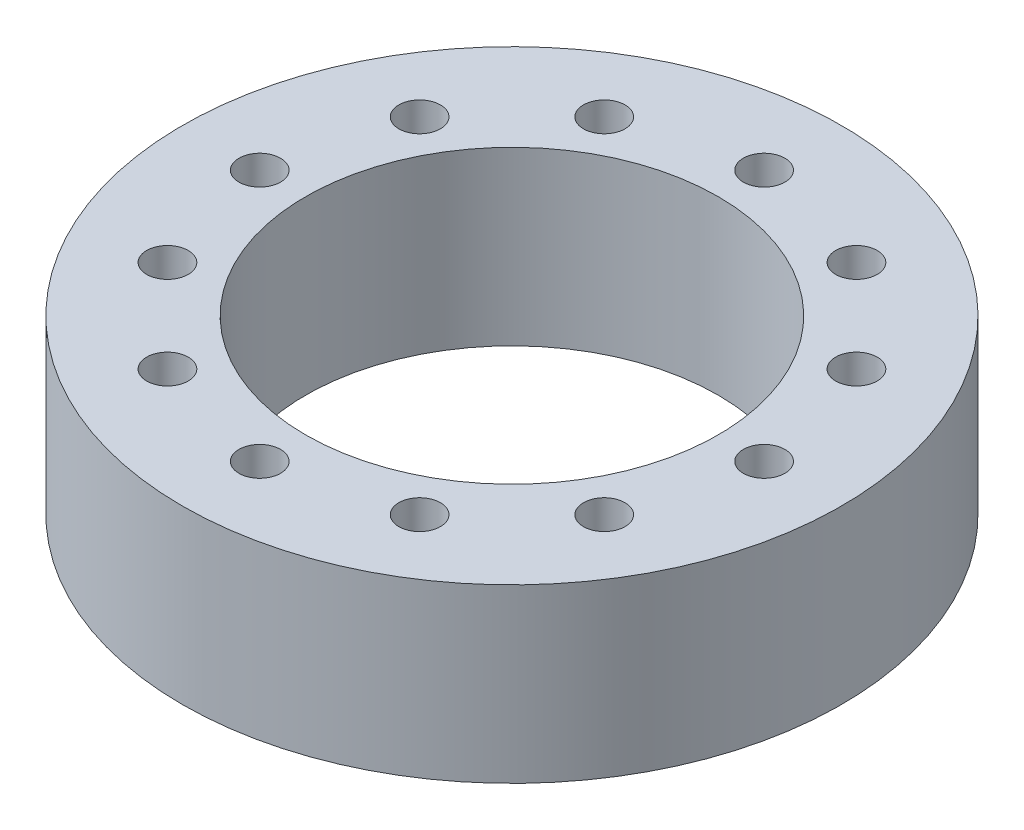
from build123d import *

# Parameters (mm, degrees)
SKETCH1_R           = 115
SKETCH1_R_2         = 72
SKETCH1_R_3         = 7.25
BOSS_EXTRUDE1_DEPTH = 60
SKETCH2_R           = 11
CUT_EXTRUDE1_DEPTH  = 30


with BuildPart() as part:
    # Sketch1 → Boss-Extrude1 (new body)
    with BuildSketch(Plane(origin=(0, 0, 0), x_dir=(1, 0, 0), z_dir=(0, 1, 0))):
        with Locations(Location((0, 0, 0), (0, 0, 270))):
            Circle(SKETCH1_R)
        with Locations(Location((0, 0, 0), (0, 0, 270))):
            Circle(SKETCH1_R_2, mode=Mode.SUBTRACT)
        with Locations(Location((0, 88, 0), (0, 0, 270))):
            Circle(SKETCH1_R_3, mode=Mode.SUBTRACT)
        with Locations(Location((44, 76.210235533, 0), (0, 0, 270))):
            Circle(SKETCH1_R_3, mode=Mode.SUBTRACT)
        with Locations(Location((76.210235533, 44, 0), (0, 0, 270))):
            Circle(SKETCH1_R_3, mode=Mode.SUBTRACT)
        with Locations(Location((88, 0, 0), (0, 0, 270))):
            Circle(SKETCH1_R_3, mode=Mode.SUBTRACT)
        with Locations(Location((76.210235533, -44, 0), (0, 0, 270))):
            Circle(SKETCH1_R_3, mode=Mode.SUBTRACT)
        with Locations(Location((44, -76.210235533, 0), (0, 0, 270))):
            Circle(SKETCH1_R_3, mode=Mode.SUBTRACT)
        with Locations(Location((0, -88, 0), (0, 0, 270))):
            Circle(SKETCH1_R_3, mode=Mode.SUBTRACT)
        with Locations(Location((-44, -76.210235533, 0), (0, 0, 270))):
            Circle(SKETCH1_R_3, mode=Mode.SUBTRACT)
        with Locations(Location((-76.210235533, -44, 0), (0, 0, 270))):
            Circle(SKETCH1_R_3, mode=Mode.SUBTRACT)
        with Locations(Location((-88, 0, 0), (0, 0, 270))):
            Circle(SKETCH1_R_3, mode=Mode.SUBTRACT)
        with Locations(Location((-76.210235533, 44, 0), (0, 0, 270))):
            Circle(SKETCH1_R_3, mode=Mode.SUBTRACT)
        with Locations(Location((-44, 76.210235533, 0), (0, 0, 270))):
            Circle(SKETCH1_R_3, mode=Mode.SUBTRACT)
    extrude(amount=BOSS_EXTRUDE1_DEPTH)

    # Sketch2 → Cut-Extrude1 (cut)
    with BuildSketch(Plane.XZ):
        with Locations(Location((0, 88, 0), (0, 0, 270))):
            Circle(SKETCH2_R)
        with Locations(Location((44, 76.210235533, 0), (0, 0, 270))):
            Circle(SKETCH2_R)
        with Locations(Location((76.210235533, 44, 0), (0, 0, 270))):
            Circle(SKETCH2_R)
        with Locations(Location((88, 0, 0), (0, 0, 270))):
            Circle(SKETCH2_R)
        with Locations(Location((76.210235533, -44, 0), (0, 0, 270))):
            Circle(SKETCH2_R)
        with Locations(Location((44, -76.210235533, 0), (0, 0, 270))):
            Circle(SKETCH2_R)
        with Locations(Location((0, -88, 0), (0, 0, 270))):
            Circle(SKETCH2_R)
        with Locations(Location((-44, -76.210235533, 0), (0, 0, 270))):
            Circle(SKETCH2_R)
        with Locations(Location((-76.210235533, -44, 0), (0, 0, 270))):
            Circle(SKETCH2_R)
        with Locations(Location((-88, 0, 0), (0, 0, 270))):
            Circle(SKETCH2_R)
        with Locations(Location((-76.210235533, 44, 0), (0, 0, 270))):
            Circle(SKETCH2_R)
        with Locations(Location((-44, 76.210235533, 0), (0, 0, 270))):
            Circle(SKETCH2_R)
    extrude(amount=-CUT_EXTRUDE1_DEPTH, mode=Mode.SUBTRACT)


solid = part.part
